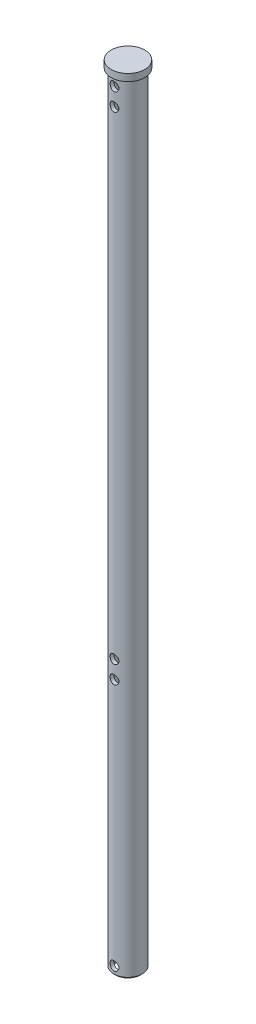
SolidWorks part; units mm, degrees
material "A3"
ref_plane "前视基准面" through (0, 0, 0) normal (0, 0, 1) x (1, 0, 0)
ref_plane "上视基准面" through (0, 0, 0) normal (0, 1, 0) x (1, 0, 0)
ref_plane "右视基准面" through (0, 0, 0) normal (1, 0, 0) x (0, 0, -1)
sketch "草图1" plane through (0, 0, 0) normal (0, 1, 0) x (1, 0, 0)
  circle A0 centre (0, 0) radius 19
  dimension "D1" = 38
extrude "凸台-拉伸1" add sketch "草图1" along normal blind 8
sketch "草图2" plane through (0, 0, 0) normal (0, -1, 0) x (1, 0, 0)
  circle A0 centre (0, 0) radius 16
  circle A1 centre (0, 0) radius 12
  dimension "D1" = 32
  dimension "D2" = 24
extrude "凸台-拉伸2" add sketch "草图2" along normal blind 880
ref_plane "基准面1" through (-16, 0, 0) normal (-1, 0, 0) x (0, 0, 1)
chamfer "倒角1" distance 2 angle 45 1 edges at (0, -880, -16)
sketch "草图10" plane through (0, 0, 0) normal (0, 0, 1) x (1, 0, 0)
  line L0 (-14, -880) -> (14, -880) construction
  line L1 (0, 0) -> (0, -880) construction
  circle A0 centre (0, -870) radius 5
  circle A1 centre (0, -590) radius 5
  circle A2 centre (0, -570) radius 5
  circle A3 centre (0, -30) radius 5
  circle A4 centre (0, -10) radius 5
  dimension "D1" = 10
  dimension "D3" = 10
  dimension "D5" = 540
  dimension "D6" = 20
  dimension "D2" = 10
  dimension "D4" = 20
extrude "切除-拉伸2" cut sketch "草图10" against normal through all both and the other way through all
